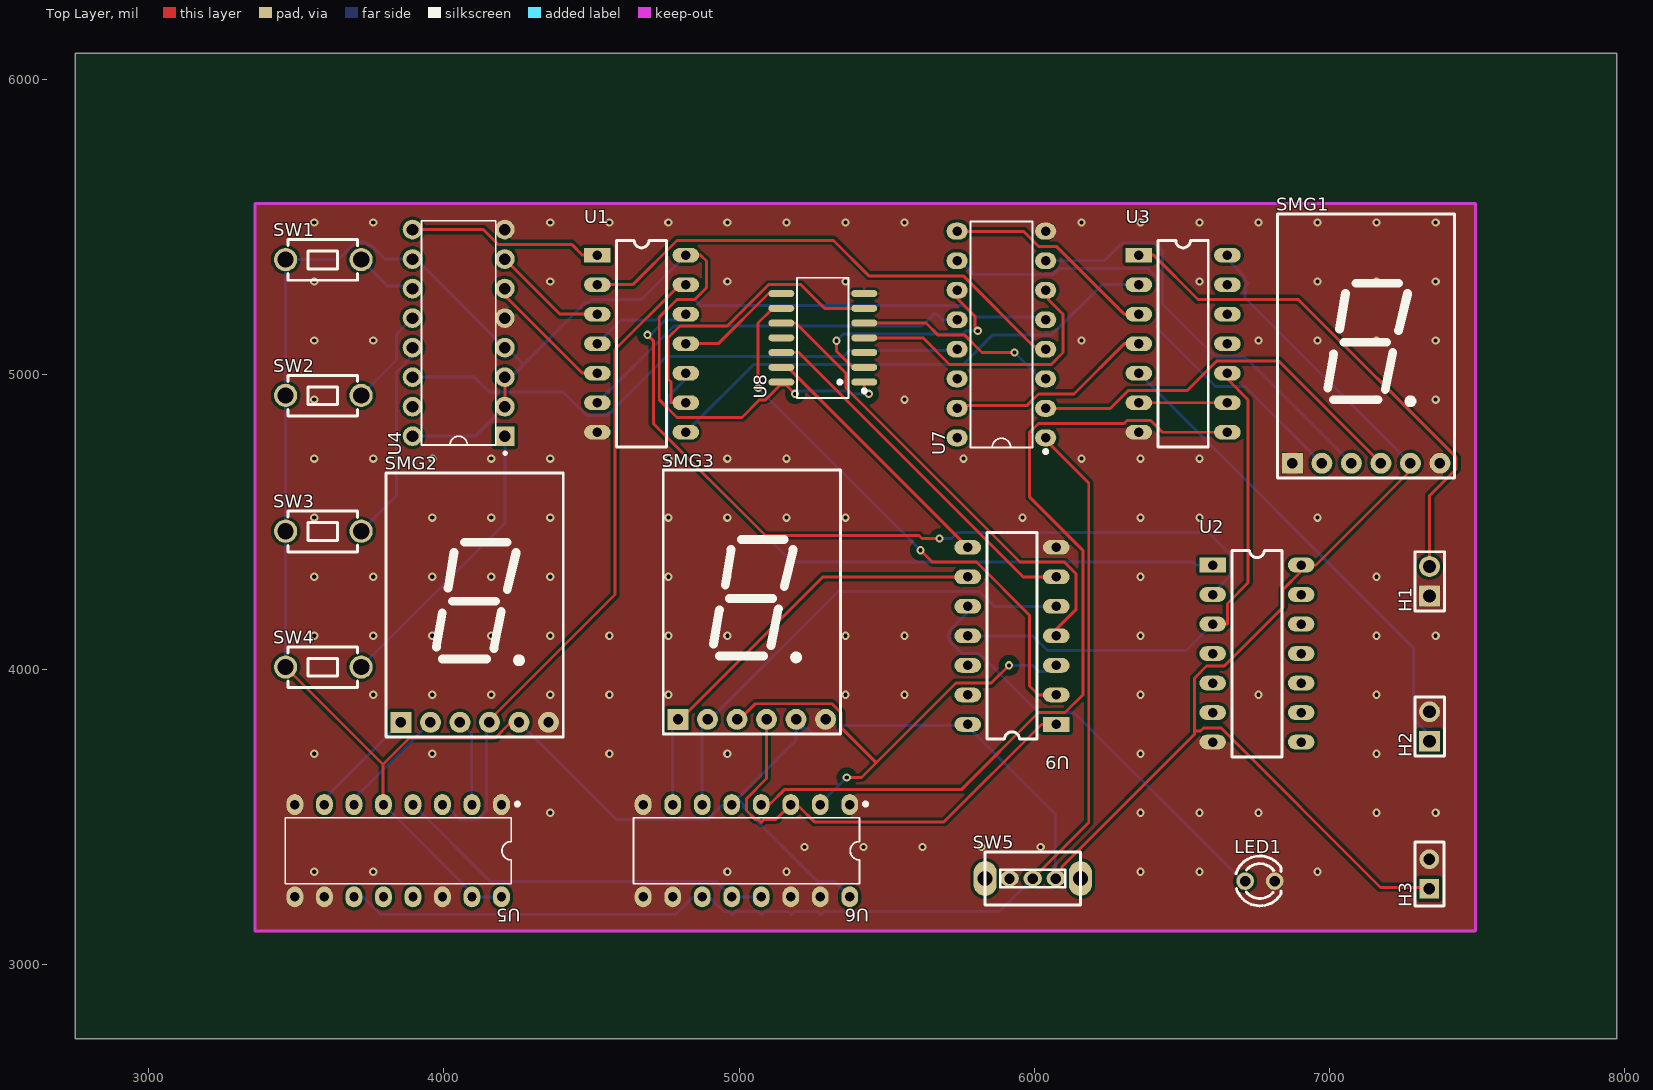
[diagram p0: Top Layer view]
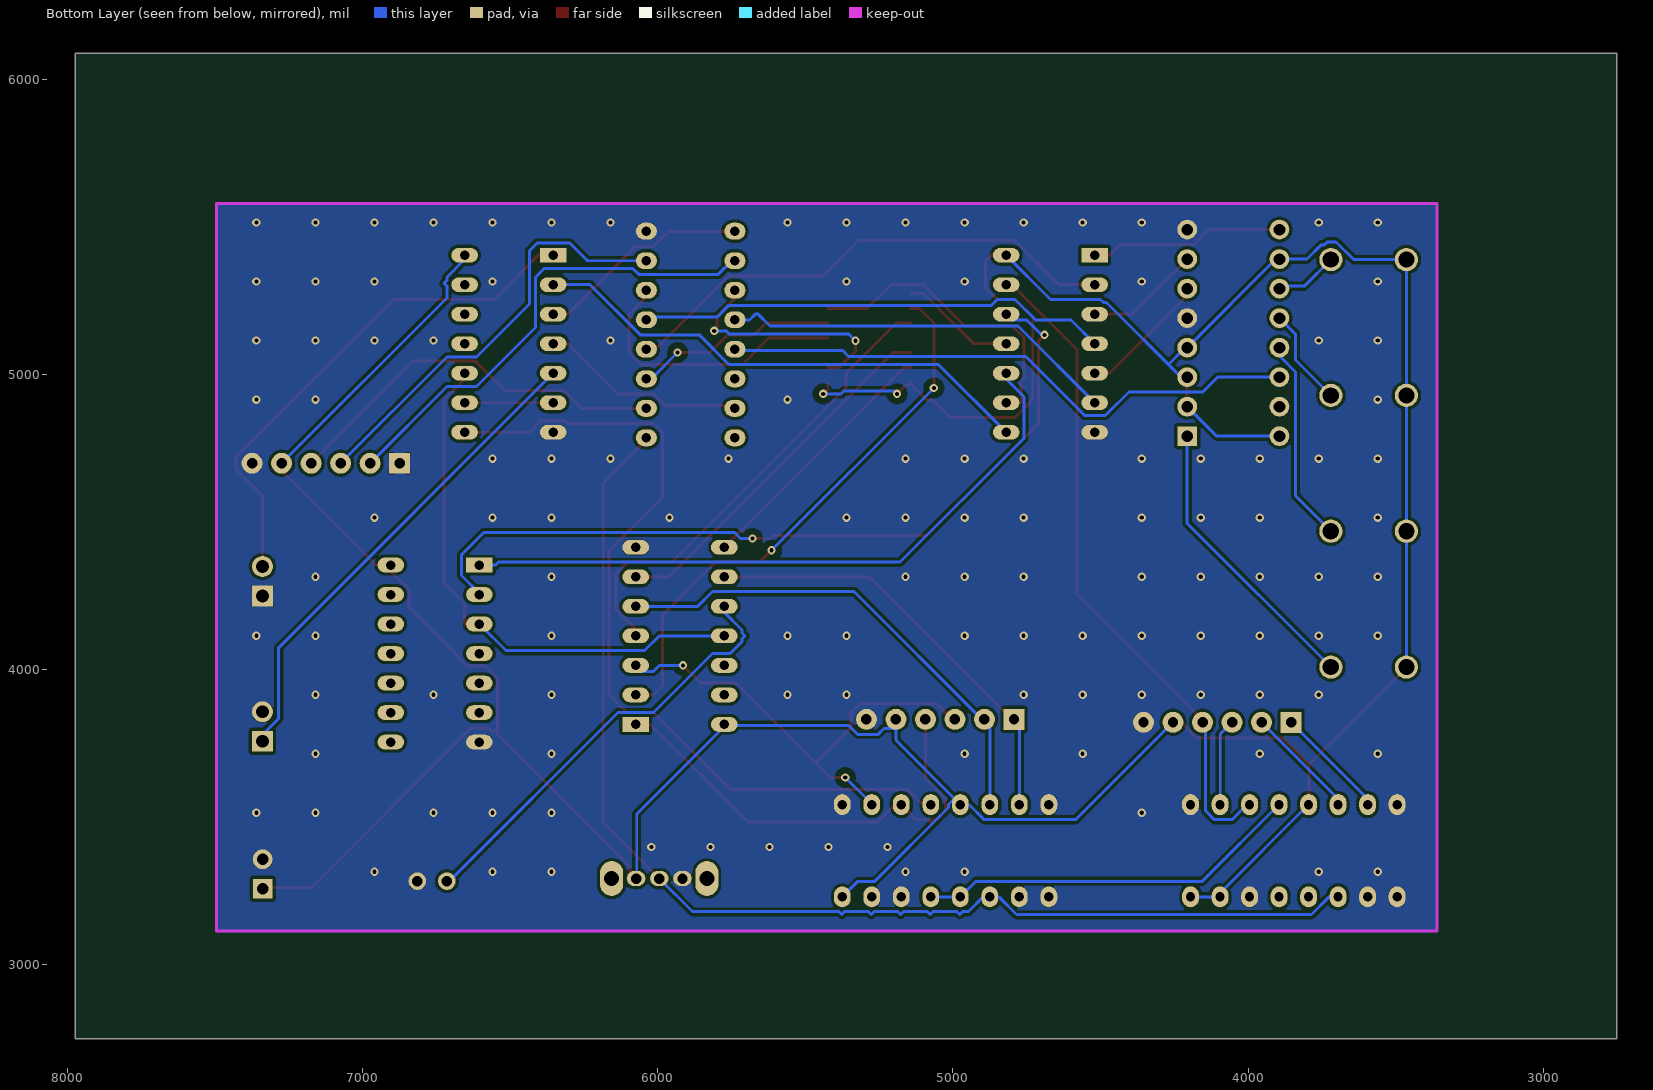
[diagram p1: Bottom Layer view, seen from below]
# Altium PCB MISC52149.pcbdoc
Units mil, origin at the board's own origin, x right, y up, seen from the top; angles counter-clockwise.
Board outline 5225 x 3340 mil, 2 copper layers (Top Layer, Bottom Layer); 21 components, 46 nets, 173 pads, 128 vias.

## Layer stack, top to bottom (the 12.6 mil dielectric is the usual default, probably not edited)
Top Solder Mask Layer: solder mask 0.4, Solder Resist, Dk 3.5
Top Layer: signal copper 1.4
Dielectric 1: surface 12.6, FR-4, Dk 4.8
Bottom Layer: signal copper 1.4
Bottom Solder Mask Layer: solder mask 0.4, Solder Resist, Dk 3.5

## Board outline
7975,2750 2750,2750 2750,6090 7975,6090

## Design rules (kind name [scope] priority, off if disabled: settings)
BoardOutlineClearance Plane_PlaneConnect_1 [All] p2 off: genericclearance=10 ignorepadtopadclearanceinfootprint=FALSE except(0: Poly-OutlineEdge Poly-CutoutEdge Arc-SplitContinuation Track-SplitContinuation SMDPad-SplitContinuation THPad-SplitContinuation Via-SplitContinuation Fill-SplitContinuation Region-SplitContinuation Poly-SplitContinuation Text-SplitContinuation Hole-SplitContinuation; 10: Arc-OutlineEdge Track-OutlineEdge SMDPad-OutlineEdge THPad-OutlineEdge Via-OutlineEdge Fill-OutlineEdge Region-OutlineEdge Text-OutlineEdge Hole-OutlineEdge Arc-CutoutEdge Track-CutoutEdge SMDPad-CutoutEdge THPad-CutoutEdge Via-CutoutEdge Fill-CutoutEdge Region-CutoutEdge Text-CutoutEdge Hole-CutoutEdge)
BoardOutlineClearance Copper_PolygonConnect_1 [All] p4 off: genericclearance=10 ignorepadtopadclearanceinfootprint=FALSE except(0: Poly-OutlineEdge Poly-CutoutEdge Arc-SplitContinuation Track-SplitContinuation SMDPad-SplitContinuation THPad-SplitContinuation Via-SplitContinuation Fill-SplitContinuation Region-SplitContinuation Poly-SplitContinuation Text-SplitContinuation Hole-SplitContinuation; 10: Arc-OutlineEdge Track-OutlineEdge SMDPad-OutlineEdge THPad-OutlineEdge Via-OutlineEdge Fill-OutlineEdge Region-OutlineEdge Text-OutlineEdge Hole-OutlineEdge Arc-CutoutEdge Track-CutoutEdge SMDPad-CutoutEdge THPad-CutoutEdge Via-CutoutEdge Fill-CutoutEdge Region-CutoutEdge Text-CutoutEdge Hole-CutoutEdge)
BoardOutlineClearance Clearance_1 [All] p6: genericclearance=10 ignorepadtopadclearanceinfootprint=FALSE except(0: Arc-SplitContinuation Track-SplitContinuation SMDPad-SplitContinuation THPad-SplitContinuation Via-SplitContinuation Fill-SplitContinuation Region-SplitContinuation Poly-SplitContinuation Text-SplitContinuation Hole-SplitContinuation; 10: Arc-OutlineEdge Track-OutlineEdge SMDPad-OutlineEdge THPad-OutlineEdge Via-OutlineEdge Fill-OutlineEdge Region-OutlineEdge Poly-OutlineEdge Text-OutlineEdge Hole-OutlineEdge Arc-CutoutEdge Track-CutoutEdge SMDPad-CutoutEdge THPad-CutoutEdge Via-CutoutEdge Fill-CutoutEdge Region-CutoutEdge Poly-CutoutEdge Text-CutoutEdge Hole-CutoutEdge)
Clearance Plane_PlaneConnect [All] p1 off: gap=10 ignorepadtopadclearanceinfootprint=FALSE except(0: Hole-Track Hole-SMDPad Hole-THPad Hole-Via Fill-Hole Region-Hole Hole-Arc Hole-Text; 6: Poly-Track Poly-SMDPad Poly-THPad Poly-Via Poly-Fill Poly-Region Poly-Poly Poly-Arc Poly-Text Poly-Hole)
Clearance Copper_PolygonConnect [All] p3 off: gap=10 ignorepadtopadclearanceinfootprint=FALSE except(0: Hole-Track Hole-SMDPad Hole-THPad Hole-Via Fill-Hole Region-Hole Hole-Arc Hole-Text)
Clearance [All] p5: gap=10 ignorepadtopadclearanceinfootprint=FALSE except(0: Hole-Track Hole-SMDPad Hole-THPad Hole-Via Fill-Hole Region-Hole Hole-Arc Hole-Text)
DiffPairsRouting [All] p1: maxlimit=10 minlimit=10 mostfreqgap=10 toplayer_minwidth=15 toplayer_prefwidth=15 toplayer_maxwidth=15 toplayer_mingap=10 toplayer_prefgap=10 toplayer_maxgap=10 bottomlayer_minwidth=15 bottomlayer_prefwidth=15 bottomlayer_maxwidth=15 bottomlayer_mingap=10 bottomlayer_prefgap=10 bottomlayer_maxgap=10 maxuncoupledlength=500
Length netLength [All] p1: minlimit=0 maxlimit=0
MatchedLengths netLengthTolerance [All] p1: tolerance=1000
PolygonConnect [All] p1: connectstyle=Relief reliefconductorwidth=0 reliefentries=4 polygonreliefangle="90 Angle" airgapwidth=1 smdpad.connectstyle=Relief smdpad.reliefconductorwidth=10 smdpad.reliefentries=4 smdpad.polygonreliefangle="90 Angle" smdpad.airgapwidth=10 via.connectstyle=Relief via.reliefconductorwidth=10 via.reliefentries=4 via.polygonreliefangle="90 Angle" via.airgapwidth=10
RoutingVias [All] p1: holewidth=28 width=50 viastyle="Through Hole" minholewidth=1 minwidth=1 maxholewidth=28 maxwidth=50
SolderMaskExpansion [All] p1: expansion=4 istentingtop=FALSE
Width [All] p1: maxlimit=30 minlimit=10 preferedwidth=10
3 further rules are at their usual default settings.

## Components (designator, comment, footprint, x,y, rotation, side; value= is the part's Value field where it differs from the comment)
H1 "" HDR-TH_2P-P2.54-V-M-1 7340,4300 r90 top
H2 "" HDR-TH_2P-P2.54-V-M-1 7340,3807.96 r90 top
H3 "" HDR-TH_2P-P2.54-V-F 7339.21,3308.05 r90 top
LED1 "" LED_TH-3mm 6765,3283.99 r0 top
SMG1 "SMG" B含CD译码器的数码管 7130,5110 r0 top
SMG2 "SMG" B含CD译码器的数码管 4109.38,4232.13 r0 top
SMG3 "SMG" B含CD译码器的数码管 5048.28,4242.13 r0 top
SW1 "" Key_TH_3.5x6x4.3 3585,5390 r0 top
SW2 "" Key_TH_3.5x6x4.3 3585,4929.79 r0 top
SW3 "" Key_TH_3.5x6x4.3 3585,4469.58 r0 top
SW4 "" Key_TH_3.5x6x4.3 3585,4009.37 r0 top
SW5 "" 拨动开关 5990,3292.68 r0 top
U1 "74LS04" DIP-014 4654.72,5110 r0 top
U2 "74LS32" DIP-014 6740,4060 r0 top
U3 "74LS00" DIP-014 6490,5110 r0 top
U4 "SN74148N" PDIP-16_L19.3-W6.4-P2.54-LS7.9-BL 4050,5141.67 r90 top
U5 "SN74LS192N(XBLW)" PDIP-16_L19.3-W6.4-P2.54-LS7.94-BL 3845,3386.91 r180 top
U6 "SN74LS192N(XBLW)" PDIP-16_L19.3-W6.4-P2.54-LS7.94-BL 5025,3386.91 r180 top
U7 "SN74175N" DIP-16_L19.3-W6.4-P2.54-LS7.6-BL 5889.12,5136.17 r90 top
U8 "SN74LS21NS" SOIC-14_L10.0-W5.5-P1.27-LS7.8-BL 5283.96,5125 r90 top
U9 "74LS04" DIP-014 5940,4110 r180 top

## Footprints (in the part's own frame and the unit in brackets; to place one, negate y for a bottom-side part, rotate by r counter-clockwise, add the part's x,y. Pads: shape width x height; smd on the part's side, far side on the other; paste and mask are expansions set on the pad)
B含CD译码器的数码管 [mm]
  rect 1.8x1.8 hole 0.9: 1(-6.477,-10.414)
  round 1.8 hole 0.9: 2(-3.937,-10.414) 3(-1.397,-10.414) 4(1.143,-10.414) 5(3.683,-10.414) 6(6.223,-10.414)
  silkscreen extent -7.75,-11.68 7.49,11.05
DIP-014 [mil]
  rect 90x50 hole 32: 1(-135,295)
  oval 90x50 hole 32: 2(-135,195) 3(-135,95) 4(-135,-5) 5(-135,-105) 6(-135,-205) 7(-135,-305) 8(165,-305) 9(165,-205) 10(165,-105) 11(165,-5) 12(165,95) 13(165,195) 14(165,295)
  silkscreen extent -70,-355 100,345
DIP-16_L19.3-W6.4-P2.54-LS7.6-BL [mm]
  oval 1.46x1.825 hole 0.8: 1(-8.89,-3.81) 2(-6.35,-3.81) 3(-3.81,-3.81) 4(-1.27,-3.81) 5(1.27,-3.81) 6(3.81,-3.81) 7(6.35,-3.81) 8(8.89,-3.81) 9(8.89,3.81) 10(6.35,3.81) 11(3.81,3.81) 12(1.27,3.81) 13(-1.27,3.81) 14(-3.81,3.81) 15(-6.35,3.81) 16(-8.89,3.81)
  silkscreen extent -10.22,-3.96 9.73,2.67
HDR-TH_2P-P2.54-V-F [mm]
  rect 1.7x1.7 hole 1: 1(-1.27,0)
  round 1.7 hole 1: 2(1.27,0)
  silkscreen extent -2.74,-1.25 2.74,1.25
HDR-TH_2P-P2.54-V-M-1 [mm]
  rect 1.8x1.8 hole 1.1: 1(-1.27,0)
  round 1.8 hole 1.1: 2(1.27,0)
  silkscreen extent -2.54,-1.27 2.54,1.27
Key_TH_3.5x6x4.3 [mil]
  round 78.7 hole 55.1 paste+0 mask+2: A(-121.44,0) B(134.46,0)
  silkscreen extent -114,-70 123,68
LED_TH-3mm [mil]
  round 60 hole 36 paste+0 mask+2: 1(-50,0) 2(50,0)
  silkscreen extent -81,-84 72,85
PDIP-16_L19.3-W6.4-P2.54-LS7.9-BL [mm]
  rect 1.7x1.7 hole 1: 1(-8.89,-3.97)
  round 1.7 hole 1 copper offset 0,0: 2(-6.35,-3.97) 3(-3.81,-3.97) 4(-1.27,-3.97) 5(1.27,-3.97) 6(3.81,-3.97) 7(6.35,-3.97) 8(8.89,-3.97)
  round 1.7 hole 1: 9(8.89,3.97) 10(6.35,3.97) 11(3.81,3.97) 12(1.27,3.97) 13(-1.27,3.97) 14(-3.81,3.97) 15(-6.35,3.97) 16(-8.89,3.97)
  silkscreen extent -10.46,-4.1 9.65,3.2
PDIP-16_L19.3-W6.4-P2.54-LS7.94-BL [mm]
  oval 1.44x1.8 hole 0.8: 1(-8.89,-3.97) 2(-6.35,-3.97) 3(-3.81,-3.97) 4(-1.27,-3.97) 5(1.27,-3.97) 6(3.81,-3.97) 7(6.35,-3.97) 8(8.89,-3.97) 9(8.89,3.97) 10(6.35,3.97) 11(3.81,3.97) 12(1.27,3.97) 13(-1.27,3.97) 14(-3.81,3.97) 15(-6.35,3.97) 16(-8.89,3.97)
  silkscreen extent -10.41,-4.17 9.73,2.84
SOIC-14_L10.0-W5.5-P1.27-LS7.8-BL [mil]
  oval 23.7x87.83 smd: 1(-150,-140.37) 2(-100,-140.37) 3(-50,-140.37) 4(0,-140.37) 5(50,-140.37) 6(100,-140.37) 7(150,-140.37) 8(150,140.37) 9(100,140.37) 10(50,140.37) 11(0,140.37) 12(-50,140.37) 13(-100,140.37) 14(-150,140.37)
  silkscreen extent -204,-146 204,87
拨动开关 [mil]
  oval 63x51.2 hole 35.4 paste+0 mask+2: 1(-73.4,0) 2(5,0) 3(84,0)
  oval 78.7x118.1 hole 51.2 paste+0 mask+2: 4(166.7,0) 5(-156.1,0)
  silkscreen extent -156,-90 167,90

## Via types
v1: diameter 28, hole 14, Top Layer to Bottom Layer, 128 vias

## Nets (pads, with @x,y where several pads share a name; then routed paths per layer and width w, separated by ;. In a path a pad name is that pad's centre, name@x,y a point inside that pad or via, vN(x,y) a via of type N, cw(c..) or ccw(c..) an arc to the next point about the centre after c; other vN are vias at no path point)
$1N808: SW1.B U4.11 | length 215
  Bottom Layer w10: SW1.B 3809.46,5300 3885.38,5300 U4.11
$1N809: SW2.B U4.12 | length 334.1
  Bottom Layer w10: SW2.B 3839.46,5049.79 3839.46,5137.43 U4.12
$1N810: SW3.B U4.13 | length 694.3
  Bottom Layer w10: SW3.B 3839.46,4589.58 3839.46,5009.58 3889.46,5059.58 3889.46,5087.43 U4.13
$1N811: SW4.B U4.1 | length 984
  Bottom Layer w10: SW4.B 4206.3,4496.21 U4.1
$1N815: U1.1 U4.9 | length 661.9
  Top Layer w10: U4.9 4133.04,5491.67 4183.04,5441.67 4433.04,5441.67 4469.72,5405 U1.1
$1N816: U1.3 U4.7 | length 390.7
  Top Layer w10: U4.7 4392.97,5205 U1.3
$1N817: U1.5 U4.6 | length 445.2
  Top Layer w10: U4.6 4209.72,5285 4209.72,5265 4469.72,5005 U1.5
$1N818: U1.2 U7.4 | length 1734.1
  Top Layer w10: U1.2 4639.72,5305 4789.72,5455 5319.72,5455 5439.72,5335 5759.72,5335 5999.71,5095 6029.71,5095 U7.4
$1N819: U1.4 U7.5 | length 1609.9
  Bottom Layer w10: U1.4 4599.72,5185 4719.72,5185 4789.72,5255 4849.72,5255 4869.72,5235 5759.71,5235 5799.71,5195 6029.71,5195 U7.5
$1N820: U1.6 U7.12 | length 1352
  Bottom Layer w10: U1.6 4779.72,5165 5619.72,5165 5659.72,5205 5669.72,5205 5689.72,5185 5729.72,5185 U7.12
$1N821: U4.14 U7.13 | length 1992
  Bottom Layer w10: U4.14 4103.7,4991.67 4153.7,4941.67 4403.7,4941.67 4483.7,4861.67 4553.7,4861.67 4753.7,5061.67 5353.7,5061.67 5373.7,5081.67 5733.7,5081.67 U7.13
$1N822: SMG1.4 U7.2 | length 1345.5
  Top Layer w10: U7.2 6258.83,4886.17 6318.83,4946.17 6518.83,4946.17 6618.83,5046.17 6828.83,5046.17 SMG1.4
$1N823: SMG1.3 U7.7 | length 1475.2
  Bottom Layer w10: U7.7 6238.83,5386.17 6298.83,5446.17 6408.83,5446.17 6435,5420 6435,5240 6615,5060 6715,5060 SMG1.3
$1N824: SMG1.2 U7.10 | length 1636.2
  Bottom Layer w10: U7.10 5748.83,5386.17 5795,5340 6065,5340 6085,5360 6385,5360 6415,5330 6415,5160 6615,4960 6715,4960 SMG1.2
$1N825: SW5.2 U5.11 U6.11 U7.1 | length 4090.9
  Top Layer w10: SW5.2 6185,3482.68 6185,4632.67 6039.12,4778.55 U7.1
  Bottom Layer w10: U5.11 3725,3230.61 3785,3170.61 4785,3170.61 4845,3230.61 U6.11 4897.07,3230.61 4947.07,3180.61 4967.07,3180.61 4977.07,3170.61 4987.07,3180.61 5067.07,3180.61 5077.07,3170.61 5087.07,3180.61 5167.07,3180.61 5177.07,3170.61 5187.07,3180.61 5267.07,3180.61 5277.07,3170.61 5287.07,3180.61 5367.07,3180.61 5377.07,3170.61 5387.07,3180.61 5882.94,3180.61 SW5.2
$1N826: U3.3 U7.9 | length 732
  Top Layer w10: U7.9 5745,5485 5965,5485 6015,5435 6075,5435 6305,5205 U3.3
$1N829: U1.8 U3.2 | length 1742.4
  Bottom Layer w10: U1.8 5049.72,5035 5759.71,5035 5859.71,5135 6059.71,5135 6229.71,5305 U3.2
$1N830: H1.2 U3.1 | length 1766
  Top Layer w10: U3.1 6405,5405 6555,5255 6895,5255 7430,4720 7430,4680 7340,4590 H1.2
$1N832: U1.9 U8.6 | length 1046.4
  Top Layer w10: U1.9 4769.72,4905 4769.72,4975 4759.72,4985 4759.72,5125 4799.72,5165 4959.72,5165 5099.72,5305 5209.72,5305 5289.72,5225 U8.6
$1N835: U7.3 U8.5 | length 693
  Top Layer w10: U8.5 5633.16,5175 5673.16,5135 5763.16,5135 5823.16,5075 v1(5933.16,5075)
  Bottom Layer w10: v1(5933.16,5075) 6021.98,4986.17 U7.3
$1N836: U7.6 U8.4 | length 962.4
  Top Layer w10: U8.4 5623.16,5125 5713.16,5035 6057.95,5035 6097.95,5075 6097.95,5205 6047.95,5255 6047.95,5275 U7.6
$1N837: U7.11 U8.2 | length 811
  Top Layer w10: v1(5330.49,5115) 5330.49,5079.51 5385,5025 U8.2 ; U7.11 5739.12,5258.63 5799.12,5198.63 5799.12,5158.63 v1(5809.12,5148.63)
  Bottom Layer w10: v1(5330.49,5115) 5354.13,5138.63 5759.12,5138.63 5769.12,5148.63 v1(5809.12,5148.63)
$1N839: U3.4 U7.15 | length 707.1
  Top Layer w10: U7.15 5745,4885 5755,4895 5975,4895 6015,4935 6135,4935 6305,5105 U3.4
$1N842: H2.1 U3.5 | length 1654.6
  Bottom Layer w10: U3.5 7285,4075 7285,3835 7335,3785 7335,3765 H2.1
$1N843: U3.6 U3.9 | length 300
  Top Layer w10: U3.6 U3.9
$1N844: U2.3 U3.10 U9.11 | length 1846
  Top Layer w10: U2.3 6655,4155 6655,4225 6725,4295 6725,4915 6655,4985 U3.10
  Bottom Layer w10: U9.11 5995,4115 6045,4065 6515,4065 U2.3
$1N845: U1.10 U2.1 | length 2268.2
  Bottom Layer w10: U1.10 4819.72,4985 4759.72,4925 4759.72,4785 5179.72,4365 6539.71,4365 6549.71,4355 U2.1
$1N846: U1.12 U2.2 | length 2783.1
  Top Layer w10: v1(4689.72,5135) 4709.72,5115 4709.72,4835 5089.72,4455 5609.72,4455 5619.72,4445 v1(5679.72,4445)
  Bottom Layer w10: v1(4689.72,5135) 4699.72,5135 4749.72,5185 4799.72,5185 U1.12 ; v1(5679.72,4445) 5719.72,4445 5739.72,4465 6589.71,4465 6665,4389.71 6665,4319.71 6605,4259.71 U2.2
$1N847: U1.11 U8.8 | length 394.3
  Top Layer w10: U1.11 4929.72,5105 5099.72,5275 U8.8
$1N849: U8.13 U9.8 | length 884.1
  Top Layer w10: U8.13 5165,5025 U9.8
$1N850: U8.12 U9.6 | length 1246.2
  Top Layer w10: U8.12 5202.42,5075 5962.42,4315 U9.6
$1N851: U8.10 U9.4 | length 1618.1
  Top Layer w10: U8.10 5192.42,5175 5362.42,5005 5362.42,4955 5952.42,4365 6102.42,4365 6142.42,4325 6142.42,4205 6075,4137.58 U9.4
$1N852: U8.9 U9.2 | length 1901.2
  Top Layer w10: v1(5064.76,4955) 5064.76,5175 5114.76,5225 U8.9 ; v1(5614.75,4405) 5654.75,4365 5804.75,4365 5984.75,4185 5984.75,3945 6014.75,3915 U9.2
  Bottom Layer w10: v1(5064.76,4955) v1(5614.75,4405)
$1N858: SMG3.4 U6.3 U9.1 | length 1589
  Top Layer w10: SMG3.4 5093.28,3631.49 5025,3563.21 5025,3523.21 5055,3493.21 5065,3493.21 5075,3483.21 5085,3493.21 5125,3493.21 U6.3 5185,3535 5205,3535 5255,3485 5695,3485 6025,3815 U9.1
$1N859: SMG3.3 U6.2 U9.3 | length 1618.3
  Top Layer w10: SMG3.3 5002.13,3832.13 5055,3885 5315,3885 5345,3855 5345,3805 5465,3685 ; v1(5365,3635) 5415,3635 5735,3955 5855,3955 v1(5915,4015)
  Bottom Layer w10: U6.2 5285,3555 v1(5365,3635) ; v1(5915,4015) 5995,4015 6015,3995 6055,3995 U9.3
$1N860: SMG3.2 U6.6 U9.5 | length 1678.2
  Bottom Layer w10: U6.6 4875,3813.84 SMG3.2 4902.13,3832.13 5335,4265 5815,4265 5865,4215 U9.5
$1N861: SMG3.1 U6.7 U9.9 | length 1478.2
  Top Layer w10: SMG3.1 4802.13,3832.13 5285,4315 U9.9
  Bottom Layer w10: U6.7 4775,3813.84 SMG3.1
$1N864: U5.4 U6.12 U6.13 | length 1309.5
  Bottom Layer w10: U5.4 4155,3283.21 4922.4,3283.21 U6.12 U6.13
$1N868: U3.8 U6.4 | length 2911.1
  Top Layer w10: U6.4 5085,3545 5105,3545 5155,3595 5755,3595 6015,3855 6105,3855 6165,3915 6165,4405 5985,4585 5985,4805 6015,4835 6305,4835 6315,4845 6395,4845 6435,4805 U3.8
$1N869: LED1.1 U9.10 | length 1488.7
  Bottom Layer w10: U9.10 5775,4195 5715,4135 5715,4125 5705,4115 5715,4105 5715,4095 5755,4055 5815,4055 6015,3855 6135,3855 6705,3285 LED1.1
$1N871: SMG2.4 U1.13 U5.3 | length 2257.3
  Top Layer w10: SMG2.4 4154.38,3829.66 4579.72,4255 4579.72,5085 4799.72,5305 U1.13
  Bottom Layer w10: U5.3 4003.3,3543.21 4054.38,3492.13 4114.38,3492.13 4144.38,3522.13 4144.38,3812.13 SMG2.4
$1N872: SMG2.3 U5.2 | length 295.5
  Bottom Layer w10: SMG2.3 4094.38,3782.13 4094.38,3552.13 U5.2
$1N873: SMG2.2 U5.6 | length 386.4
  Bottom Layer w10: U5.6 3695,3562.75 SMG2.2
$1N874: SMG2.1 U5.7 | length 386.4
  Bottom Layer w10: U5.7 3595,3562.75 SMG2.1
GND: H1.1 H2.2 H3.2 LED1.2 SMG1.1 SMG1.6 SMG2.6 SMG3.6 SW5.1 U1.7 U2.7 U3.7 U4.5 U4.8 U5.1 U5.8 U5.9 U5.10 U5.14 U6.1 U6.8 U6.9 U6.10 U6.14 U6.15 U7.8 U8.7 U9.7
  other v1: 3560.5,3315.5 3760.5,3315.5 4960.5,3315.5 5160.5,3315.5 6360.5,3315.5 6560.5,3315.5 6960.5,3315.5 5222.01,3399.71 5422.01,3399.71 5622.01,3399.71 5822.01,3399.71 6022.01,3399.71 4360.5,3515.5 6360.5,3515.5 6560.5,3515.5 6760.5,3515.5 7160.5,3515.5 7360.5,3515.5 3560.5,3715.5 3960.5,3715.5 4560.5,3715.5 4960.5,3715.5 6360.5,3715.5 7160.5,3715.5 3760.5,3915.5 3960.5,3915.5 4160.5,3915.5 4360.5,3915.5 4560.5,3915.5 4760.5,3915.5 5360.5,3915.5 5560.5,3915.5 6360.5,3915.5 6760.5,3915.5 7160.5,3915.5 3560.5,4115.5 3760.5,4115.5 3960.5,4115.5 4160.5,4115.5 4360.5,4115.5 4560.5,4115.5 4760.5,4115.5 4960.5,4115.5 5360.5,4115.5 5560.5,4115.5 6360.5,4115.5 7160.5,4115.5 7360.5,4115.5 3560.5,4315.5 3760.5,4315.5 3960.5,4315.5 4160.5,4315.5 4360.5,4315.5 4760.5,4315.5 4960.5,4315.5 5160.5,4315.5 6360.5,4315.5 7160.5,4315.5 3560.5,4515.5 3960.5,4515.5 4160.5,4515.5 4360.5,4515.5 4760.5,4515.5 4960.5,4515.5 5160.5,4515.5 5360.5,4515.5 5960.5,4515.5 6360.5,4515.5 6560.5,4515.5 6960.5,4515.5 3560.5,4715.5 3760.5,4715.5 3960.5,4715.5 4160.5,4715.5 4360.5,4715.5 4760.5,4715.5 4960.5,4715.5 5160.5,4715.5 5760.5,4715.5 6160.5,4715.5 6360.5,4715.5 6560.5,4715.5 3560.5,4915.5 5560.5,4915.5 7160.5,4915.5 7360.5,4915.5 3560.5,5115.5 3760.5,5115.5 6160.5,5115.5 6760.5,5115.5 6960.5,5115.5 7160.5,5115.5 7360.5,5115.5 3560.5,5315.5 4360.5,5315.5 4960.5,5315.5 5360.5,5315.5 6560.5,5315.5 6960.5,5315.5 7160.5,5315.5 7360.5,5315.5 3560.5,5515.5 3760.5,5515.5 4360.5,5515.5 4560.5,5515.5 4760.5,5515.5 4960.5,5515.5 5160.5,5515.5 5360.5,5515.5 5560.5,5515.5 6160.5,5515.5 6360.5,5515.5 6560.5,5515.5 6760.5,5515.5 6960.5,5515.5 7160.5,5515.5 7360.5,5515.5
VCC: H3.1 SMG1.5 SMG2.5 SMG3.5 SW1.A SW2.A SW3.A SW4.A SW5.3 U1.14 U2.14 U3.14 U4.2 U4.3 U4.4 U4.10 U4.16 U5.5 U5.15 U5.16 U6.5 U6.16 U8.1 U8.14 U9.14 | length 13783.3
  Top Layer w10: SW4.A 3793.56,3679.37 ; U5.5 3793.56,3549.37 3793.56,3679.37 ; U4.2 U4.3 ; SMG2.5 4243.56,3819.37 4223.56,3819.37 4173.56,3769.37 3883.56,3769.37 3793.56,3679.37 ; U1.14 4869.72,5405 4889.72,5385 4889.72,5295 4849.72,5255 4789.72,5255 4729.72,5195 4729.72,4915 4789.72,4855 5009.72,4855 5069.72,4915 5089.72,4915 U8.14@5139.72,4965 ; U8.14 5139.72,4971.13 U8.14@5139.72,4965 ; v1(5189.72,4935) 5159.72,4965 U8.14@5139.72,4965 ; U8.1 5424.33,4950.39 v1(5439.72,4935) ; SW5.3 6094,3312.68 6094,3332.68 6544,3782.68 6544,3972.68 6584,4012.68 6644,4012.68 6844,4212.67 6844,4272.67 6904,4332.67 6904,4342.67 U2.14 6955,4355 7275,4675 SMG1.5 ; 6544,3792.68 6564,3792.68 6574,3802.68 6634,3802.68 7174,3262.68 7334,3262.68 H3.1@7339.21,3258.05
  Bottom Layer w10: SW4.A SW3.A SW2.A SW1.A 3642.03,5390 3702.03,5450 3732.03,5450 3742.03,5440 3752.03,5440 3800.36,5391.67 U4.10 3906.3,5391.67 U4.4 4212.97,5085 4219.72,5085 4269.72,5035 ; U5.5 4095,3243.21 U5.15 U5.16 ; U4.16 4106.3,4791.67 U4.2 ; U4.3 4209.72,4995 4229.72,4995 4479.72,5245 4489.72,5245 4499.72,5255 4669.72,5255 U1.14 ; SMG2.5 4584.38,3492.13 4894.38,3492.13 4944.38,3542.13 4974.38,3542.13 U6.5 5193.28,3761.49 SMG3.5 ; U6.5@4995,3563.21 5015,3543.21 5015,3533.21 5265,3283.21 5322.4,3283.21 U6.16 ; v1(5189.72,4935) 5199.72,4945 5369.72,4945 5379.72,4935 v1(5439.72,4935) ; SMG3.5@5193.28,3801.49 5233.28,3801.49 5253.28,3781.49 5323.28,3781.49 5353.28,3811.49 U9.14@5771.49,3811.49 ; U9.14 U9.14@5771.49,3811.49 ; SW5.3 6071.49,3295.19 6071.49,3511.49 U9.14@5771.49,3811.49 ; U3.14 6655,5390 6715,5330 6715,5320 6725,5310 6715,5300 6715,5260 SMG1.5
pads on no net: SW5.4 SW5.5 U2.4 U2.5 U2.6 U2.8 U2.9 U2.10 U2.11 U2.12 U2.13 U3.11 U3.12 U3.13 U4.15 U5.12 U5.13 U7.14 U7.16 U8.3 U8.11 U9.12 U9.13

## Polygon pours and split planes (outlines as drawn)
GND on Top Layer (solid, remove dead copper, pour order 0): 3000,5840 3000,3000 7670,3000 7670,5840
GND on Bottom Layer (solid, remove dead copper, pour order 2): 3180,5740 3180,3020 7725,3020 7725,5740

## Keep-outs
Board Outline Layer:
  lines w10: 3360,3115 3360,5580 7495,5580 7495,3115 3360,3115